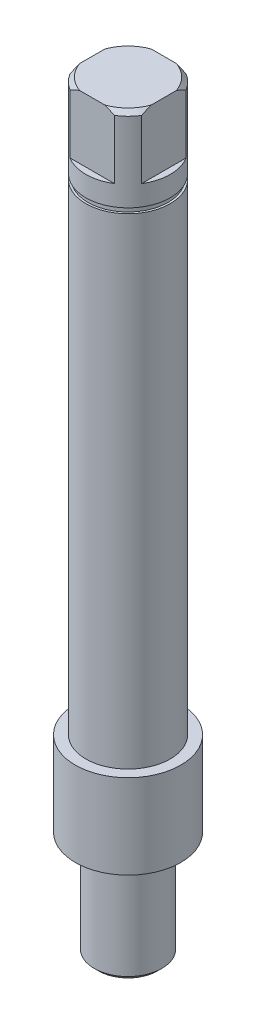
SolidWorks part; units mm, degrees
material "普通碳钢"
ref_plane "Front Plane" through (0, 0, 0) normal (0, 0, 1) x (1, 0, 0)
ref_plane "Top Plane" through (0, 0, 0) normal (0, 1, 0) x (1, 0, 0)
ref_plane "Right Plane" through (0, 0, 0) normal (1, 0, 0) x (0, 0, -1)
sketch "Sketch1" plane through (0, 0, 0) normal (0, 0, 1) x (1, 0, 0)
  line L0 (0, 0) -> (0, 110.5534) construction
  line L1 (0, 180) -> (10, 180)
  line L2 (10, 180) -> (10, 45)
  line L3 (0, 0) -> (0, 180)
  line L4 (10, 45) -> (12.5, 45)
  line L5 (12.5, 45) -> (12.5, 25)
  line L6 (8, 0) -> (0, 0)
  line L7 (8, 0) -> (8, 25)
  line L8 (8, 25) -> (12.5, 25)
  dimension "D1" = 25
  dimension "D2" = 20
  dimension "D3" = 16
  dimension "D4" = 180
  dimension "D5" = 25
  dimension "D6" = 20
revolve "Revolve1" add sketch "Sketch1" angle 360 about L0
cosmetic thread "Cosmetic Thread1" parameters "D2"=13.835
chamfer "Chamfer1" distance 1 angle 45 2 edges at (0, 180, -10) (0, 0, -8)
sketch "Sketch3" plane through (0, 0, 0) normal (0, 0, 1) x (1, 0, 0)
  line L0 (9, 180) -> (-9, 180) construction
  line L1 (-15.2992, 160.2) -> (-9.5, 160.2)
  line L2 (-15.2992, 160.2) -> (-15.2992, 159)
  line L3 (-15.2992, 159) -> (-9.5, 159)
  line L4 (-9.5, 160.2) -> (-9.5, 159)
  line L5 (0, 180) -> (0, 93.2632) construction
  dimension "D1" = 19.8
  dimension "D2" = 1.2
  dimension "D3" = 19
revolve "Cut-Revolve1" cut sketch "Sketch3" angle 360 about L5
sketch "Sketch6" plane through (0, 0, 0) normal (0, 0, 1) x (1, 0, 0)
  line L0 (0, 0) -> (0, 45) construction
  line L1 (-18.6444, 37) -> (-11, 37)
  line L2 (-18.6444, 37) -> (-18.6444, 17)
  line L3 (-18.6444, 17) -> (-11, 17)
  line L4 (-11, 37) -> (-11, 17)
  line L5 (12.5, 45) -> (-12.5, 45) construction
  line L6 (11, 37) -> (11, 17)
  line L7 (18.6444, 17) -> (11, 17)
  line L8 (18.6444, 37) -> (18.6444, 17)
  line L9 (18.6444, 37) -> (11, 37)
  line L10 (-12.5, 25) -> (12.5, 25) construction
  dimension "D1" = 22
  dimension "D2" = 12
  dimension "D3" = 20
extrude "Cut-Extrude1" [suppressed] cut sketch "Sketch6" against normal through all both and the other way through all
sketch "Sketch7" plane through (0, 0, 0) normal (0, 0, 1) x (1, 0, 0)
  line L0 (0, 180) -> (0, 117.1123) construction
  line L1 (-21.1495, 207.4276) -> (-8.5, 207.4276)
  line L2 (-21.1495, 207.4276) -> (-21.1495, 165)
  line L3 (-21.1495, 165) -> (-8.5, 165)
  line L4 (-8.5, 207.4276) -> (-8.5, 165)
  line L5 (9, 180) -> (-9, 180) construction
  line L6 (8.5, 207.4276) -> (8.5, 165)
  line L7 (21.1495, 165) -> (8.5, 165)
  line L8 (21.1495, 207.4276) -> (21.1495, 165)
  line L9 (21.1495, 207.4276) -> (8.5, 207.4276)
  dimension "D1" = 17
  dimension "D2" = 15
extrude "Cut-Extrude2" cut sketch "Sketch7" against normal through all both and the other way through all
sketch "Sketch8" plane through (0, 0, 0) normal (1, 0, 0) x (0, 0, -1)
  line L0 (0, 180) -> (0, 117.5592) construction
  line L1 (-14.1036, 208.9775) -> (-8.5, 208.9775)
  line L2 (-14.1036, 208.9775) -> (-14.1036, 165)
  line L3 (-14.1036, 165) -> (-8.5, 165)
  line L4 (-8.5, 208.9775) -> (-8.5, 165)
  line L5 (8.5, 208.9775) -> (8.5, 165)
  line L6 (14.1036, 165) -> (8.5, 165)
  line L7 (14.1036, 208.9775) -> (14.1036, 165)
  line L8 (14.1036, 208.9775) -> (8.5, 208.9775)
  line L9 (5.2678, 165) -> (8.5, 165) construction
  line L10 (2.958, 180) -> (-2.958, 180) construction
  dimension "D1" = 17
extrude "Cut-Extrude3" cut sketch "Sketch8" against normal through all both and the other way through all
